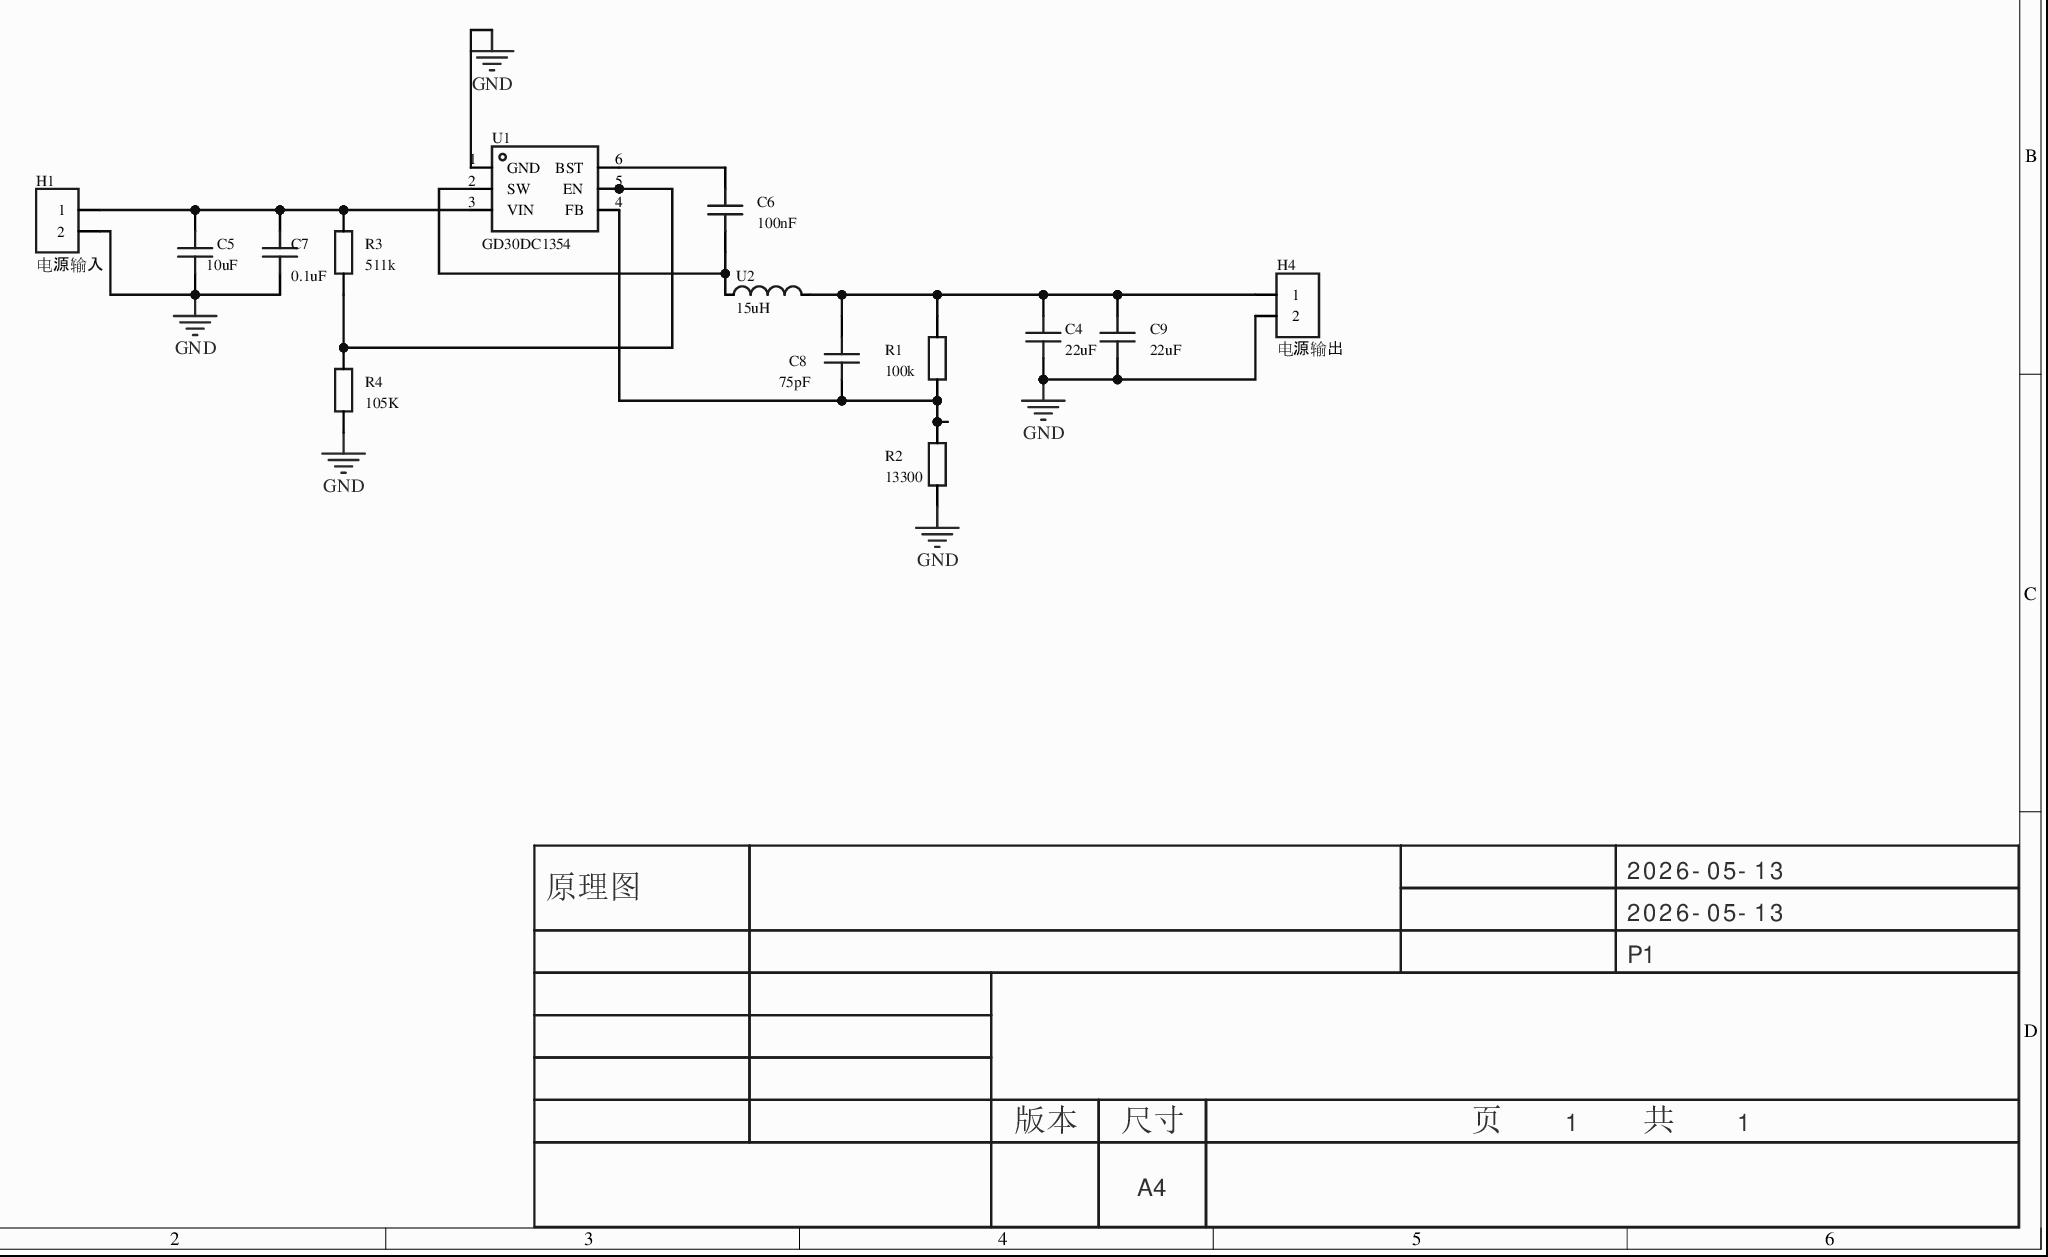
[diagram p0: MISC52146-3.schdoc]
# Altium project MISC52146-2.PrjPcb
1 sheet, 14 parts. Net scope: global (net labels, ports and power ports of the same name join across sheets).
Board file: MISC52146.pcbdoc

## Sheet MISC52146-3.schdoc
size 297 x 209 mm; Version: V1.0; @Project Name: MISC52146; @Page Count: 1; @Update Date: 2026-05-13; @Create Date: 2026-05-13; @Schematic Name: MISC52146; @Page No: 1; @Board Name: MISC52146; @Create Time: 23:17:50; @Update Time: 23:17:50; Size: A4

### Parts
C4  22uF  [C0805]
C5  10uF  [C0805]
C6  100nF  [C0805]
C7  0.1uF  [C0805]
C8  75pF  [C0805]
C9  22uF  [C0805]
H1  电源输入  [HDR-TH_2P-P2.54-V-F]
H4  电源输出  [HDR-TH_2P-P2.54-V-F]
R1  100k  [R0805]
R2  13300  [R0805]
R3  511k  [R0805]
R4  105K  [R0805]
U1  GD30DC1354  [SOT-23-6_L2.9-W1.7-P0.95-LS2.8-BL]
U2  15uH  [IND-SMD_L6.6-W6.6]

### Nets
GND: C4.1 C5.2 C7.1 C9.1 H1.2 H4.2 R2.1 R4.1 U1.1(GND)
NetC4_2: C4.2 C8.2 C9.2 H4.1 R1.2 U2.2
NetC5_1: C5.1 C7.2 H1.1 R3.1 U1.3(VIN)
NetC6_1: C6.1 U1.2(SW) U2.1
NetC6_2: C6.2 U1.6(BST)
NetC8_1: C8.1 R1.1 R2.2 U1.4(FB)
NetR3_2: R3.2 R4.2 U1.5(EN)

### Notes on the sheet
- 2026-05-13
- 原理图
- P1
- 版本
- 尺寸
- A4
- 页    1    共    1

### Library data of the parts
C4-C9 = CAP_0805: ConvertToPcb: yes; SymbolName: Capacitance; ModelId: 1ba041120af144c991958decab20d241; ModelName: C0805_L2.0-W1.3-H1.3; ModelTransform: 78.74,51.181,0,0,0,0,0,0.0005,0; Device: CAP_0805; AddInBom: yes; Supplier Footprint: 0805; FootprintName: C0805
  C4 C9: Value: 22uF
  C5: Value: 10uF
  C6: Value: 100nF
  C7: Value: 0.1uF
  C8: Value: 75pF
H1 H4 = HDR-F_2.54_1x2P: Symbol: Header-Female-2.54_1x2; ConvertToPcb: yes; ModelId: a9450ef445564560a104363b9aacde4e; ModelName: HDR-TH_2P-P2.54-F-LI-1X2P; ModelTransform: 215.7476,98.425,0,0,0,0,0,0,-129.921; Device: HDR-F_2.54_1x2P; AddInBom: yes; SupplierPart: C49661; Supplier Footprint: 插件; FootprintName: HDR-TH_2P-P2.54-V-F
R1-R4 = Res_0805: ConvertToPcb: yes; SymbolName: 电阻; ModelId: 37a81e68749a4138bd2dfa6897b24b85; ModelName: R0805_L2.0-W1.3-H0.6; ModelTransform: 78.74,51.181,0,0,0,0,0,-0.0005,0; Device: Res_0805; AddInBom: yes; Supplier Footprint: 0805; FootprintName: R0805
  R1: Value: 100k
  R2: Value: 13300
  R3: Value: 511k
  R4: Value: 105K
U1 = GD30DC1354: AddInBom: yes; ModelId: f198fe6923cc4b1fabccb73198a22cca; ModelTransform: 114.173,110.236,0,0,0,0,0,0,0; Symbol: GD30DC1354; Device: GD30DC1354; LCSC Part Name: GD30DC1354; SupplierPart: C9900263753; ManufacturerPart: GD30DC1354; Supplier Footprint: SOT23-6; Supplier: LCSC; ConvertToPcb: yes; FootprintName: SOT-23-6_L2.9-W1.7-P0.95-LS2.8-BL; ModelName: SOT-23-6_L2.9-W1.7-P0.95-LS2.8-BL
U2 = 15uH: AddInBom: yes; ModelId: 484d62df9f9b401e85d563d919dc12a20819f05c4eef4c71ace90d822a990e87; ModelTransform: 275.59,259.88137,0,0,0,0,0,0,0; Symbol: 15UH; Device: 15uH; LCSC Part Name: 15uH; SupplierPart: C9900014578; ManufacturerPart: 15uH; Supplier Footprint: L_电感_7*7; JLCPCB Part Class: Extended Part; Supplier: LCSC; ConvertToPcb: yes; FootprintName: IND-SMD_L6.6-W6.6; ModelName: IND-SMD_L6.6-W6.6